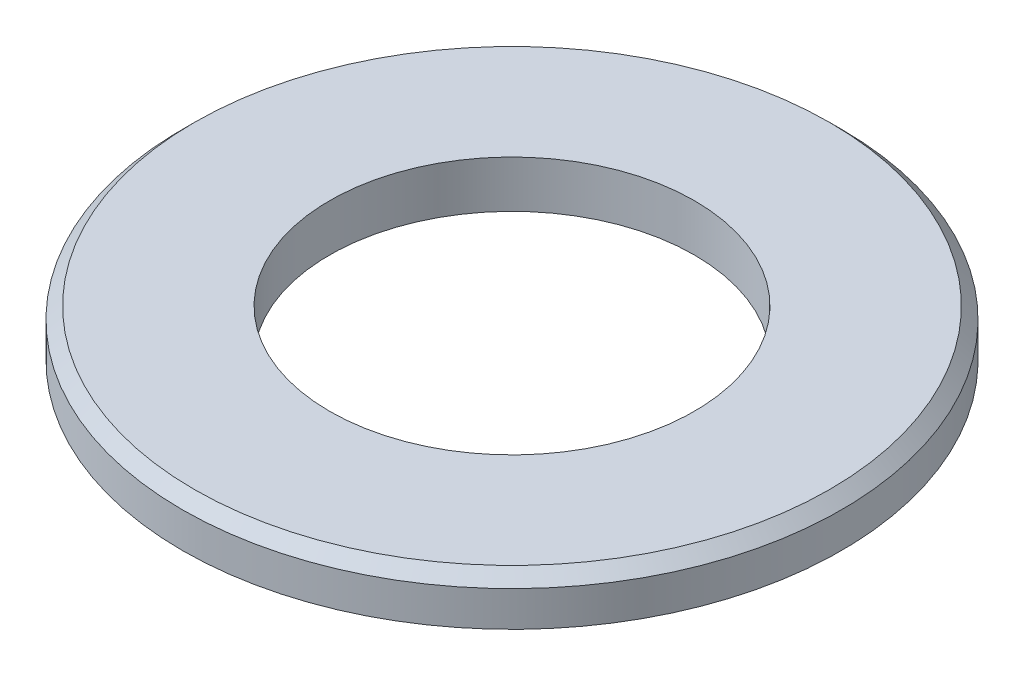
from build123d import *


with BuildPart() as part:
    # Sketch1 → Base-Revolve (revolve)
    with BuildSketch(Plane.XY, mode=Mode.PRIVATE) as base_revolve_sk:
        Polygon((-27, 12.644507042), (-28, 11.644507042), (-28, 8.644507042), (-15.5, 8.644507042), (-15.5, 12.644507042), align=None)
    revolve(base_revolve_sk.sketch.rotate(Axis((0, 0, 0), (0, 1, 0)), 270), axis=Axis((0, 0, 0), (0, 1, 0)))


solid = part.part
